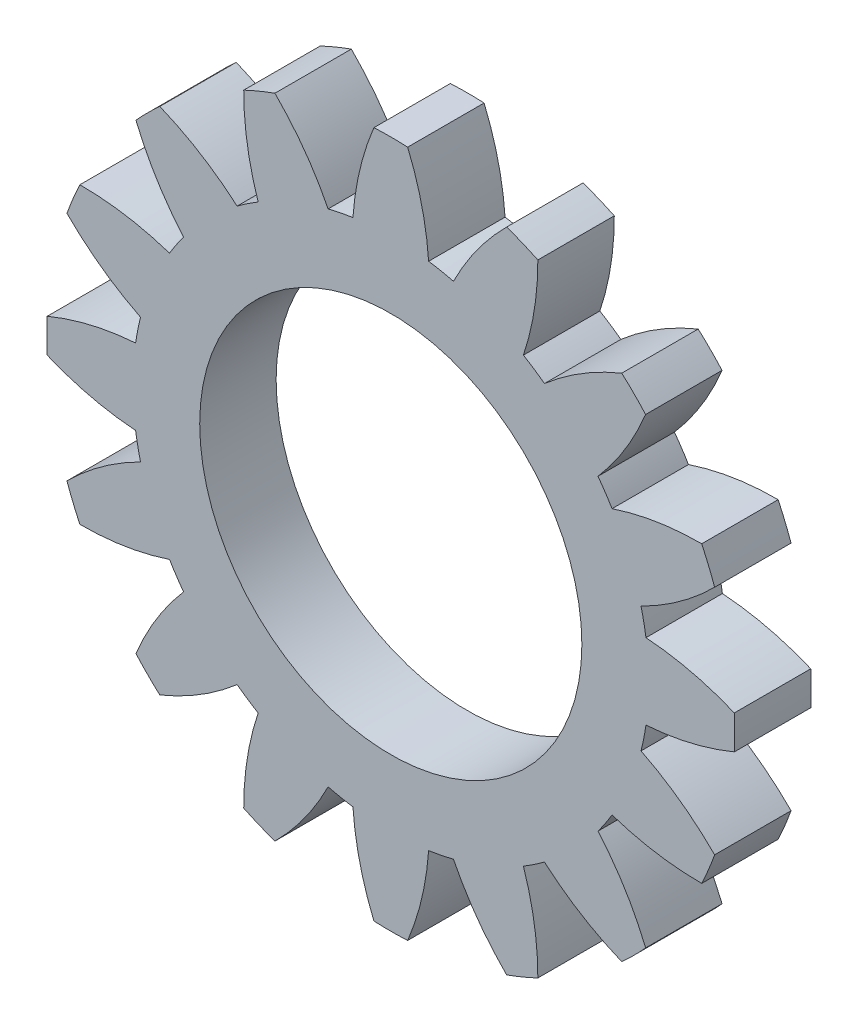
SolidWorks part; units mm, degrees
ref_plane "Front Plane" through (0, 0, 0) normal (0, 0, 1) x (1, 0, 0)
ref_plane "Top Plane" through (0, 0, 0) normal (0, 1, 0) x (1, 0, 0)
ref_plane "Right Plane" through (0, 0, 0) normal (1, 0, 0) x (0, 0, -1)
ref_plane "Plane1" through (0, 0, 0) normal (0, 0, -1) x (-1, 0, 0)
sketch "Sketch1" plane through (0, 0, 0) normal (0, 0, -1) x (-1, 0, 0)
  circle A0 centre (0, 0) radius 10
  arc A1 (6.9404, 11.5793) -> (7.696, 16.2718) centre (-6.9943, 16.2302) ccw
  arc A2 (7.696, 16.2718) -> (6.064, 16.9478) centre (0, 0) ccw
  arc A3 (6.064, 16.9478) -> (3.2802, 13.0954) centre (16.4222, 6.5308) ccw
  arc A4 (3.2802, 13.0954) -> (1.9809, 13.3539) centre (0, 0) ccw
  arc A5 (1.9809, 13.3539) -> (0.8832, 17.9783) centre (-12.6729, 12.3182) ccw
  arc A6 (0.8832, 17.9783) -> (-0.8832, 17.9783) centre (0, 0) ccw
  arc A7 (-0.8832, 17.9783) -> (-1.9809, 13.3539) centre (12.6729, 12.3182) ccw
  arc A8 (-1.9809, 13.3539) -> (-3.2802, 13.0954) centre (0, 0) ccw
  arc A9 (-3.2802, 13.0954) -> (-6.064, 16.9478) centre (-16.4222, 6.5308) ccw
  arc A10 (-6.064, 16.9478) -> (-7.696, 16.2718) centre (0, 0) ccw
  arc A11 (-7.696, 16.2718) -> (-6.9404, 11.5793) centre (6.9943, 16.2302) ccw
  arc A12 (-6.9404, 11.5793) -> (-8.0419, 10.8433) centre (0, 0) ccw
  arc A13 (-8.0419, 10.8433) -> (-12.0881, 13.3371) centre (-17.6714, -0.2508) ccw
  arc A14 (-12.0881, 13.3371) -> (-13.3371, 12.0881) centre (0, 0) ccw
  arc A15 (-13.3371, 12.0881) -> (-10.8433, 8.0419) centre (0.2508, 17.6714) ccw
  arc A16 (-10.8433, 8.0419) -> (-11.5793, 6.9404) centre (0, 0) ccw
  arc A17 (-11.5793, 6.9404) -> (-16.2718, 7.696) centre (-16.2302, -6.9943) ccw
  arc A18 (-16.2718, 7.696) -> (-16.9478, 6.064) centre (0, 0) ccw
  arc A19 (-16.9478, 6.064) -> (-13.0954, 3.2802) centre (-6.5308, 16.4222) ccw
  arc A20 (-13.0954, 3.2802) -> (-13.3539, 1.9809) centre (0, 0) ccw
  arc A21 (-13.3539, 1.9809) -> (-17.9783, 0.8832) centre (-12.3182, -12.6729) ccw
  arc A22 (-17.9783, 0.8832) -> (-17.9783, -0.8832) centre (0, 0) ccw
  arc A23 (-17.9783, -0.8832) -> (-13.3539, -1.9809) centre (-12.3182, 12.6729) ccw
  arc A24 (-13.3539, -1.9809) -> (-13.0954, -3.2802) centre (0, 0) ccw
  arc A25 (-13.0954, -3.2802) -> (-16.9478, -6.064) centre (-6.5308, -16.4222) ccw
  arc A26 (-16.9478, -6.064) -> (-16.2718, -7.696) centre (0, 0) ccw
  arc A27 (-16.2718, -7.696) -> (-11.5793, -6.9404) centre (-16.2302, 6.9943) ccw
  arc A28 (-11.5793, -6.9404) -> (-10.8433, -8.0419) centre (0, 0) ccw
  arc A29 (-10.8433, -8.0419) -> (-13.3371, -12.0881) centre (0.2508, -17.6714) ccw
  arc A30 (-13.3371, -12.0881) -> (-12.0881, -13.3371) centre (0, 0) ccw
  arc A31 (-12.0881, -13.3371) -> (-8.0419, -10.8433) centre (-17.6714, 0.2508) ccw
  arc A32 (-8.0419, -10.8433) -> (-6.9404, -11.5793) centre (0, 0) ccw
  arc A33 (-6.9404, -11.5793) -> (-7.696, -16.2718) centre (6.9943, -16.2302) ccw
  arc A34 (-7.696, -16.2718) -> (-6.064, -16.9478) centre (0, 0) ccw
  arc A35 (-6.064, -16.9478) -> (-3.2802, -13.0954) centre (-16.4222, -6.5308) ccw
  arc A36 (-3.2802, -13.0954) -> (-1.9809, -13.3539) centre (0, 0) ccw
  arc A37 (-1.9809, -13.3539) -> (-0.8832, -17.9783) centre (12.6729, -12.3182) ccw
  arc A38 (-0.8832, -17.9783) -> (0.8832, -17.9783) centre (0, 0) ccw
  arc A39 (0.8832, -17.9783) -> (1.9809, -13.3539) centre (-12.6729, -12.3182) ccw
  arc A40 (1.9809, -13.3539) -> (3.2802, -13.0954) centre (0, 0) ccw
  arc A41 (3.2802, -13.0954) -> (6.064, -16.9478) centre (16.4222, -6.5308) ccw
  arc A42 (6.064, -16.9478) -> (7.696, -16.2718) centre (0, 0) ccw
  arc A43 (7.696, -16.2718) -> (6.9404, -11.5793) centre (-6.9943, -16.2302) ccw
  arc A44 (6.9404, -11.5793) -> (8.0419, -10.8433) centre (0, 0) ccw
  arc A45 (8.0419, -10.8433) -> (12.0881, -13.3371) centre (17.6714, 0.2508) ccw
  arc A46 (12.0881, -13.3371) -> (13.3371, -12.0881) centre (0, 0) ccw
  arc A47 (13.3371, -12.0881) -> (10.8433, -8.0419) centre (-0.2508, -17.6714) ccw
  arc A48 (10.8433, -8.0419) -> (11.5793, -6.9404) centre (0, 0) ccw
  arc A49 (11.5793, -6.9404) -> (16.2718, -7.696) centre (16.2302, 6.9943) ccw
  arc A50 (16.2718, -7.696) -> (16.9478, -6.064) centre (0, 0) ccw
  arc A51 (16.9478, -6.064) -> (13.0954, -3.2802) centre (6.5308, -16.4222) ccw
  arc A52 (13.0954, -3.2802) -> (13.3539, -1.9809) centre (0, 0) ccw
  arc A53 (13.3539, -1.9809) -> (17.9783, -0.8832) centre (12.3182, 12.6729) ccw
  arc A54 (17.9783, -0.8832) -> (17.9783, 0.8832) centre (0, 0) ccw
  arc A55 (17.9783, 0.8832) -> (13.3539, 1.9809) centre (12.3182, -12.6729) ccw
  arc A56 (13.3539, 1.9809) -> (13.0954, 3.2802) centre (0, 0) ccw
  arc A57 (13.0954, 3.2802) -> (16.9478, 6.064) centre (6.5308, 16.4222) ccw
  arc A58 (16.9478, 6.064) -> (16.2718, 7.696) centre (0, 0) ccw
  arc A59 (16.2718, 7.696) -> (11.5793, 6.9404) centre (16.2302, -6.9943) ccw
  arc A60 (11.5793, 6.9404) -> (10.8433, 8.0419) centre (0, 0) ccw
  arc A61 (10.8433, 8.0419) -> (13.3371, 12.0881) centre (-0.2508, 17.6714) ccw
  arc A62 (13.3371, 12.0881) -> (12.0881, 13.3371) centre (0, 0) ccw
  arc A63 (12.0881, 13.3371) -> (8.0419, 10.8433) centre (17.6714, -0.2508) ccw
  arc A64 (8.0419, 10.8433) -> (6.9404, 11.5793) centre (0, 0) ccw
extrude "Boss-Extrude1" add sketch "Sketch1" against normal blind 4
sketch "Sketch2" plane through (0, 0, 4) normal (0, 0, 1) x (1, 0, 0)
  circle A0 centre (0, 0) radius 16
  dimension "D1" = 32
